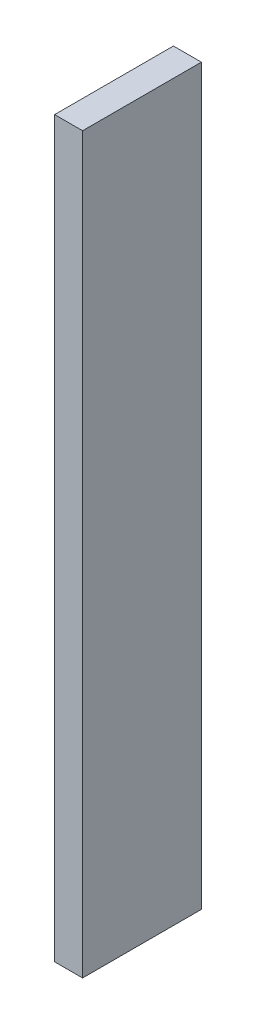
from build123d import *

# Parameters (mm, degrees)
SKETCH_1_W      = 8
SKETCH_1_H      = 210
EXTRUDE_1_DEPTH = 34


with BuildPart() as part:
    # 草图1 → 凸台-拉伸1 (new body)
    with BuildSketch(Plane.XY):
        Rectangle(SKETCH_1_W, SKETCH_1_H)
    extrude(amount=EXTRUDE_1_DEPTH)


solid = part.part
